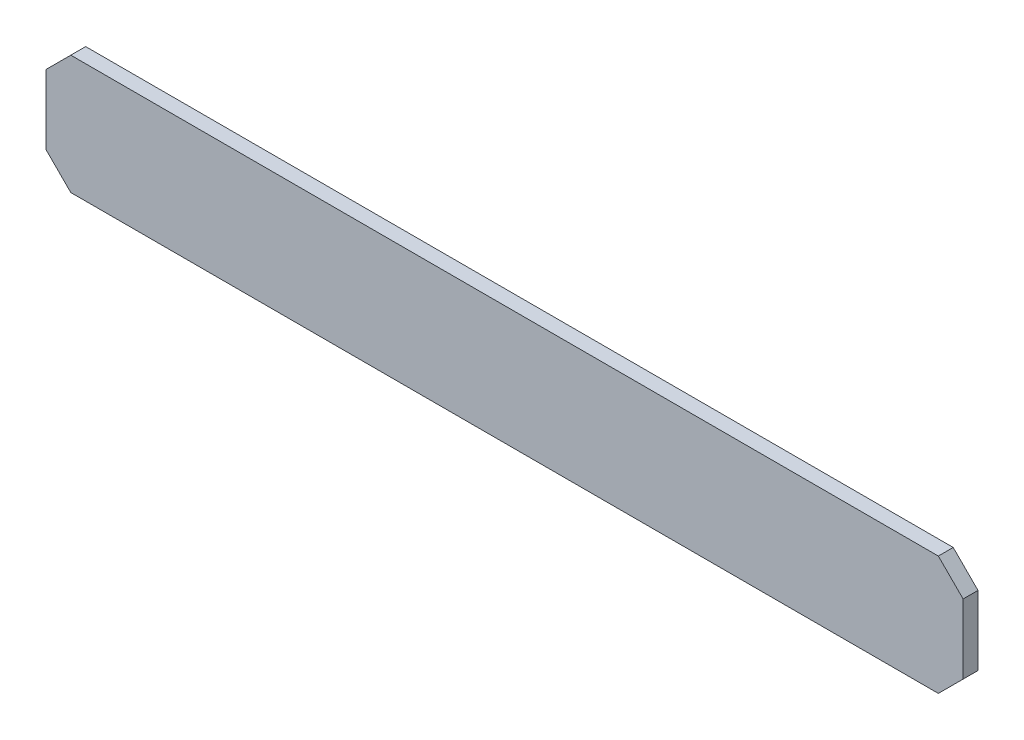
from build123d import *

# Parameters (mm, degrees)
EXTRUDE_1_DEPTH = 3


with BuildPart() as part:
    # 草图1 → 凸台-拉伸1 (new body)
    with BuildSketch(Plane.XY):
        Polygon((-92.5, 19), (-87.5, 24), (87.5, 24), (92.5, 19), (92.5, 5), (87.5, 0), (-87.5, 0), (-92.5, 5), align=None)
    extrude(amount=EXTRUDE_1_DEPTH)


solid = part.part
